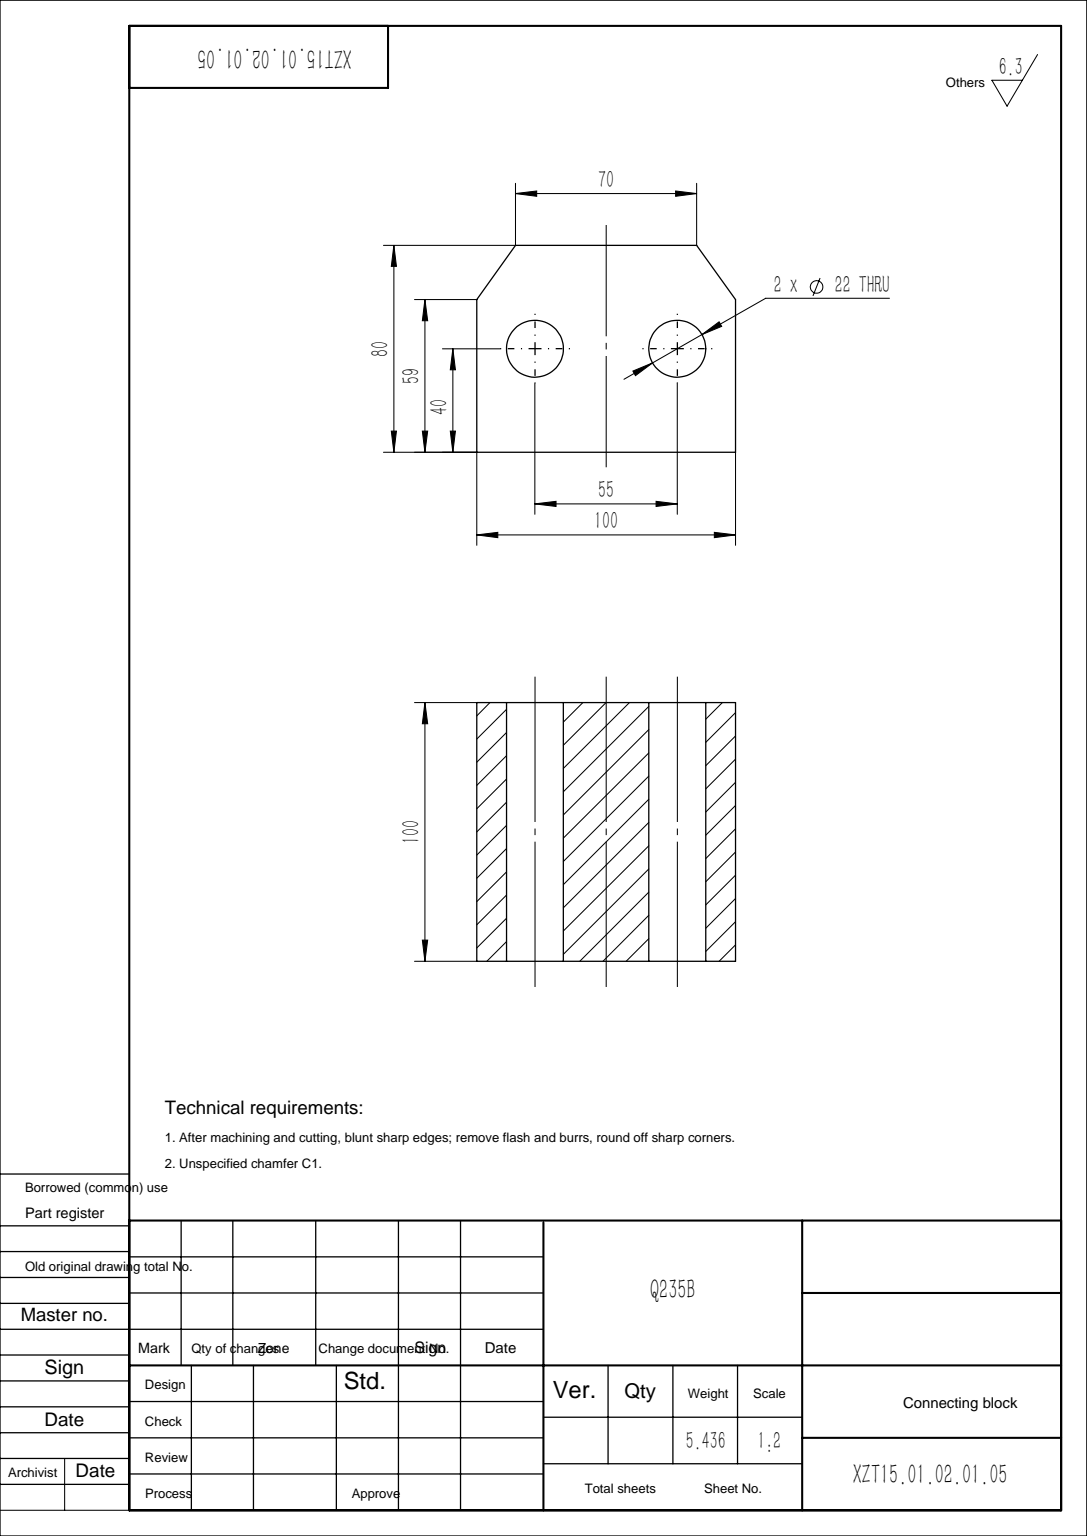
from build123d import *

# Parameters (mm, degrees)
SKETCH1_W               = 100
SKETCH1_H               = 80
BOSS_EXTRUDE1_DEPTH     = 100
CHAMFER1_SIZE           = 10
F_22_DIAMETER_HOLE1_D   = 22
CUT_EXTRUDE1_DEPTH      = 119.74342087
CUT_EXTRUDE1_DEPTH_BACK = 119.74342087


with BuildPart() as part:
    # Sketch1 → Boss-Extrude1 (new body)
    with BuildSketch(Plane.XY):
        Rectangle(SKETCH1_W, SKETCH1_H)
    extrude(amount=BOSS_EXTRUDE1_DEPTH)

    # Chamfer1
    chamfer1_edges = [part.edges().sort_by_distance(p)[0] for p in [
        (-50, 40, 50),
        (50, 40, 50),
    ]]
    chamfer(chamfer1_edges, length=CHAMFER1_SIZE)

    # Ø22 Diameter Hole1 (through all)
    with Locations(Plane.XY.offset(100)):
        with Locations((-27.5, 0), (27.5, 0)):
            Hole(F_22_DIAMETER_HOLE1_D / 2)

    # Sketch4 → Cut-Extrude1 (cut, two sides: drawn at the far end of the back side and taken through both)
    with BuildSketch(Plane.XY.offset(100).offset(-CUT_EXTRUDE1_DEPTH_BACK)):
        Polygon((-35, 40), (-50, 19), (-50, 40), align=None)
        Polygon((50, 40), (35, 40), (50, 19), align=None)
    extrude(amount=CUT_EXTRUDE1_DEPTH + CUT_EXTRUDE1_DEPTH_BACK, mode=Mode.SUBTRACT)


solid = part.part
